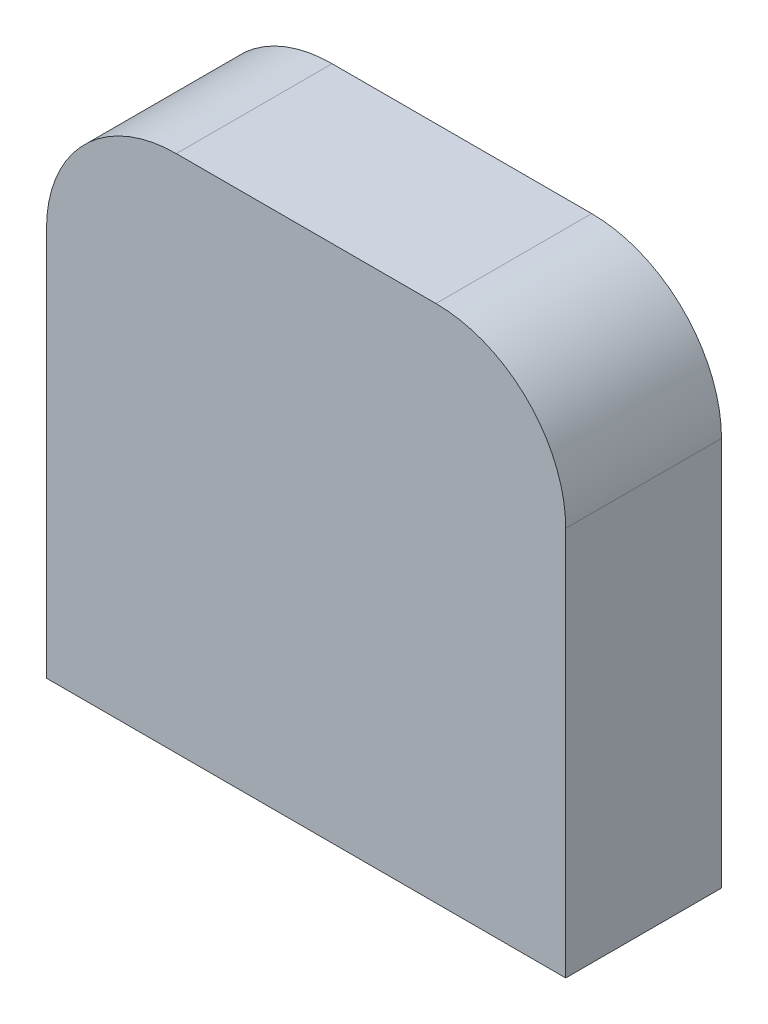
from build123d import *

# Parameters (mm, degrees)
BOSS_EXTRUDE1_DEPTH = 12


with BuildPart() as part:
    # Sketch1 → Boss-Extrude1 (new body)
    with BuildSketch(Plane.XY):
        with BuildLine():
            Line((0, 0), (40, 0))
            Line((40, 0), (40, 30))
            ThreePointArc((40, 30), (37.071067812, 37.071067812), (30, 40))
            Line((30, 40), (10, 40))
            ThreePointArc((10, 40), (2.928932188, 37.071067812), (0, 30))
            Line((0, 30), (0, 0))
        make_face()
    extrude(amount=BOSS_EXTRUDE1_DEPTH)


solid = part.part
